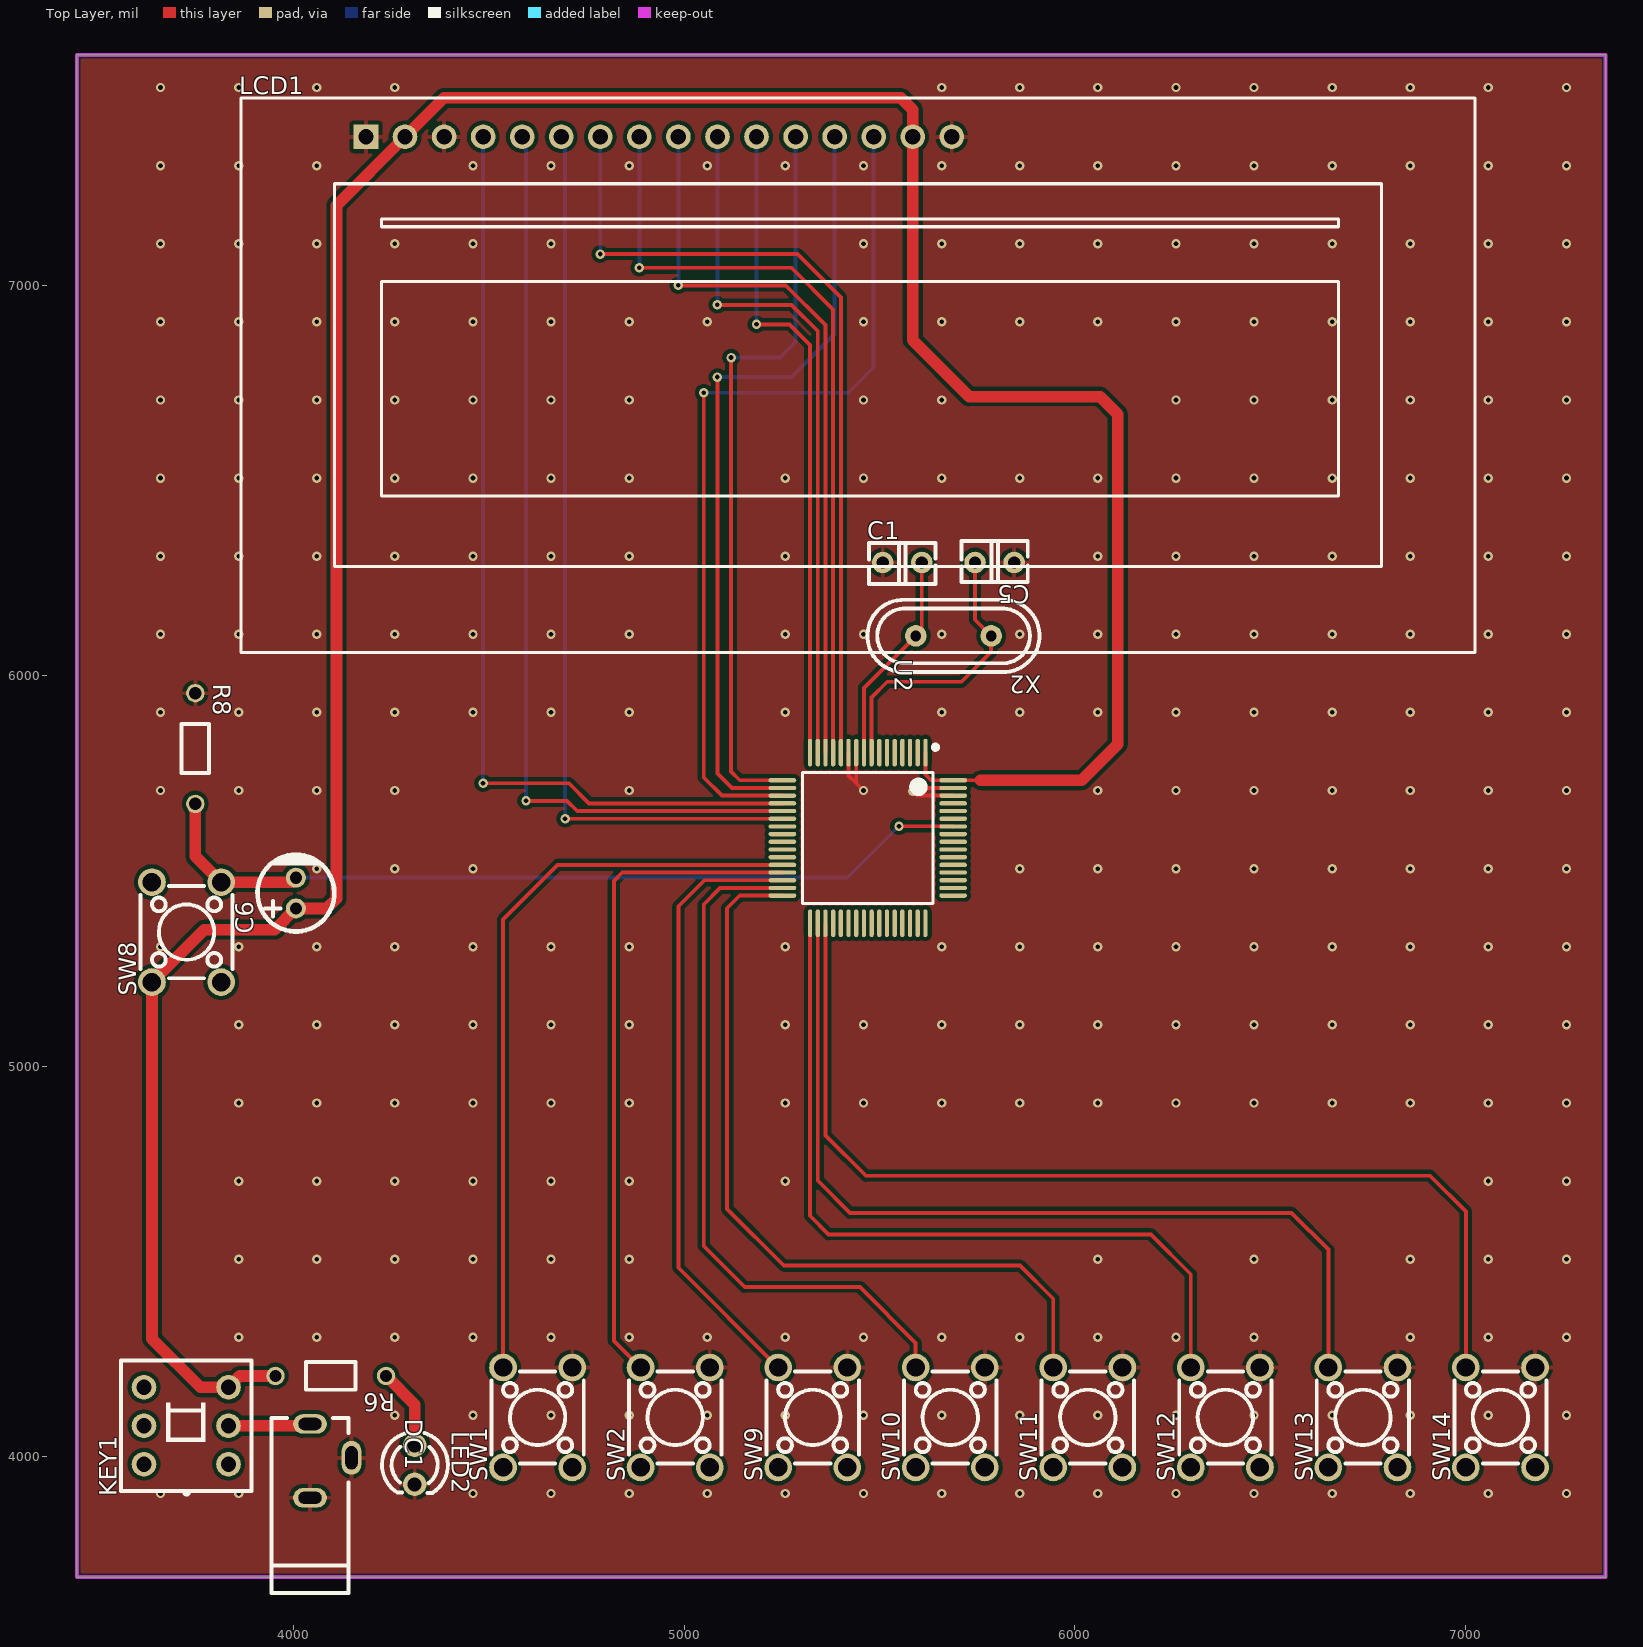
[diagram p0: Top Layer view]
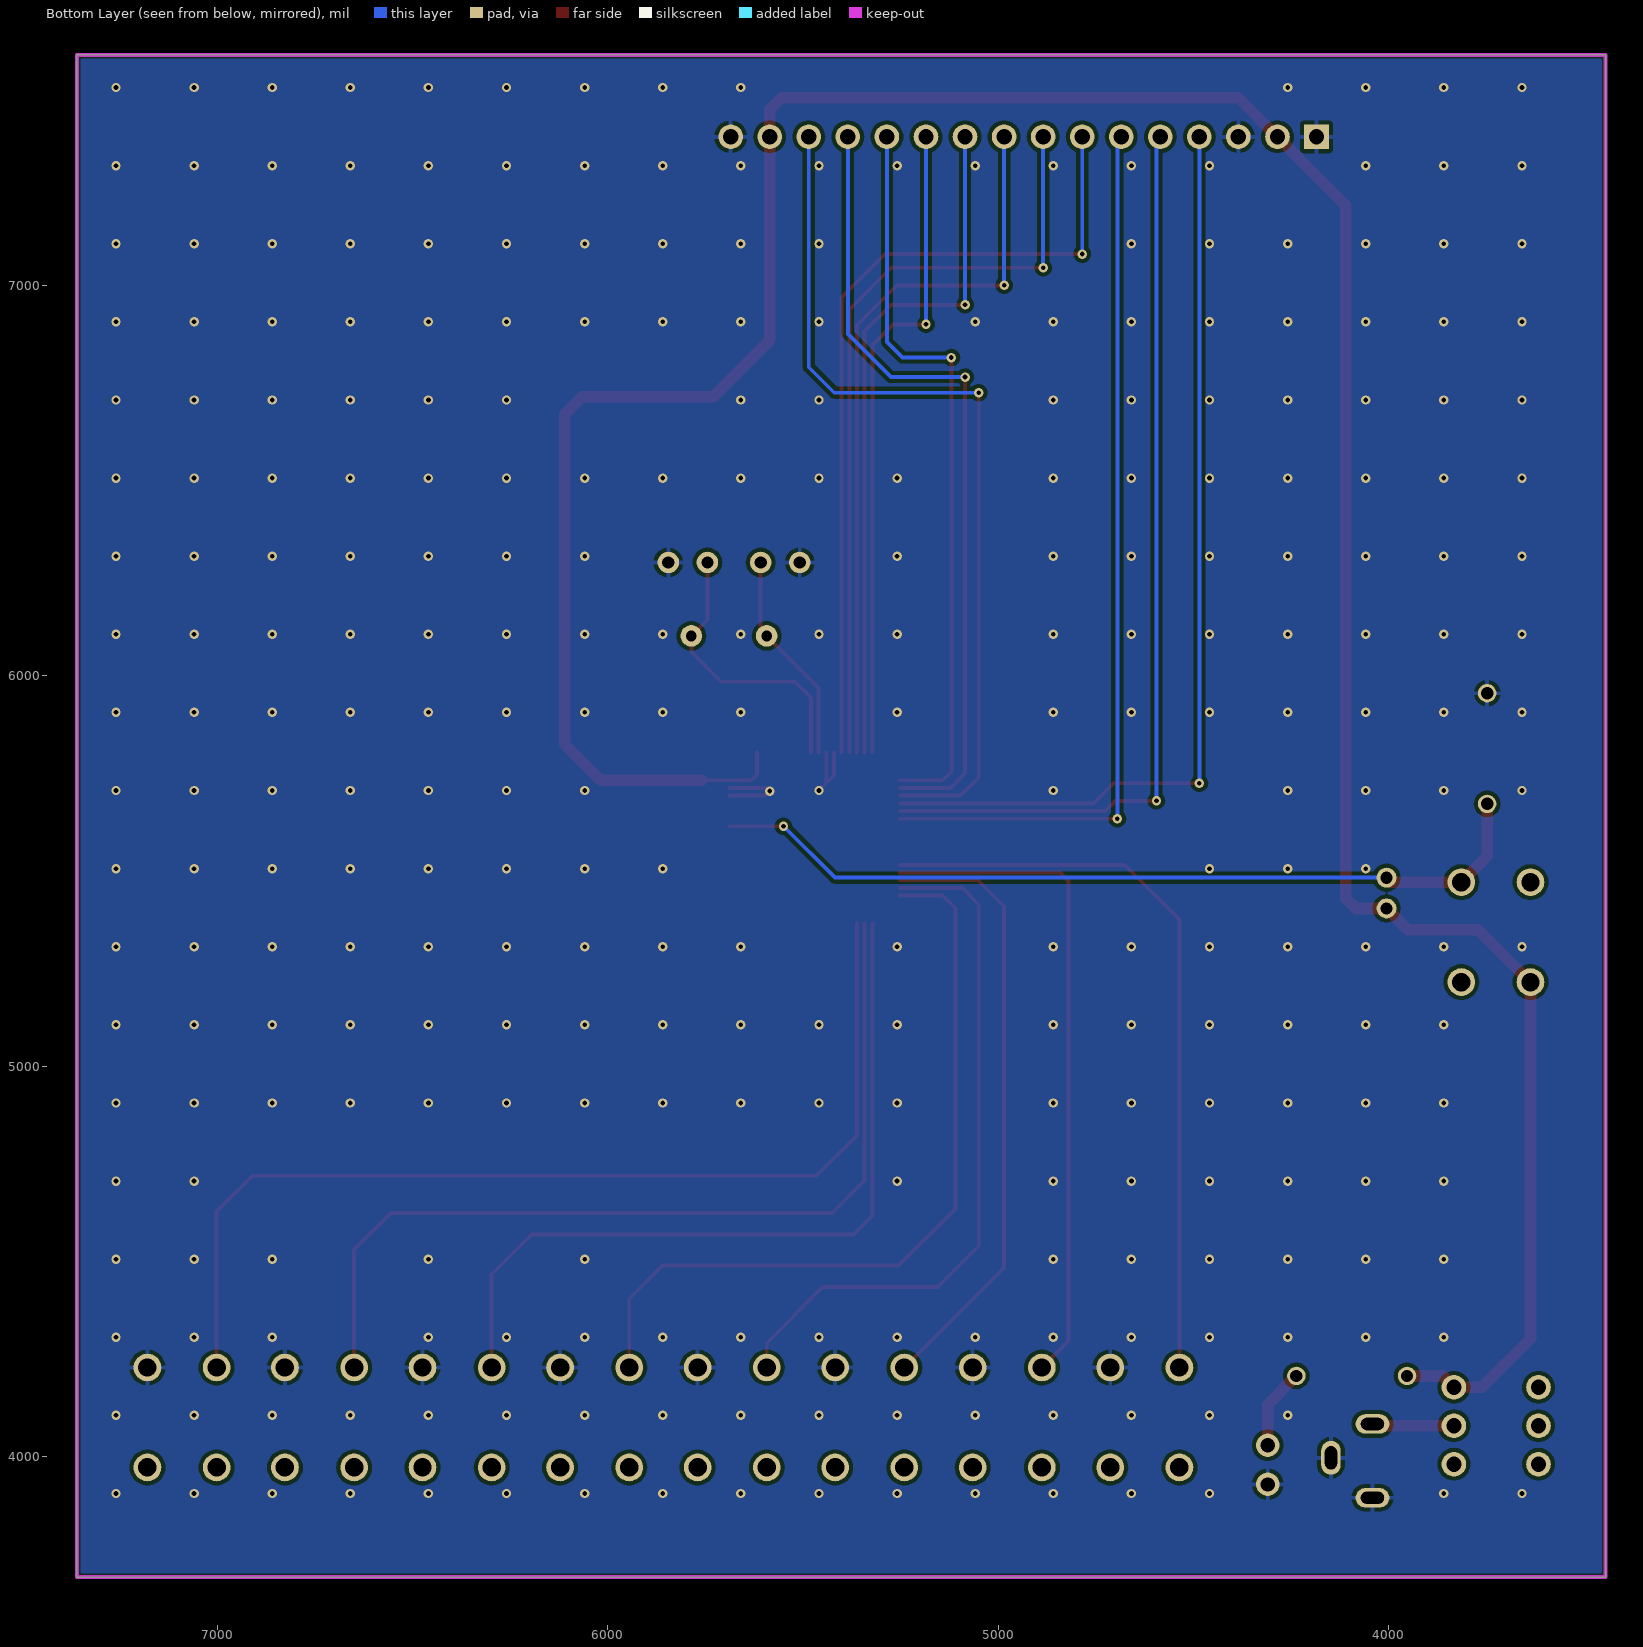
[diagram p1: Bottom Layer view, seen from below]
# Altium PCB MISC51174.pcbdoc
Units mil, origin at the board's own origin, x right, y up, seen from the top; angles counter-clockwise.
Board outline 3914.17 x 3897.64 mil, 2 copper layers (Top Layer, Bottom Layer), stack 62.206 mil thick; 20 components, 26 nets, 139 pads, 306 vias.

## Layer stack, top to bottom
Top Solder Mask Layer: solder mask 0.394, Dk 3.3
Top Layer: signal copper 1.379
Dielectric1: surface 59.449, FR4, Dk 4.5
Bottom Layer: signal copper 1.378
Bottom Solder Mask Layer: solder mask 0.394, Dk 3.3

## Board outline
3445,7590 3445,3692.36 7359.17,3692.36 7359.17,7590

## Design rules (kind name [scope] priority, off if disabled: settings)
BoardOutlineClearance copperThickness2oz_1 [All] p2 off: genericclearance=7.99 ignorepadtopadclearanceinfootprint=FALSE except(0: Arc-SplitContinuation Track-SplitContinuation SMDPad-SplitContinuation THPad-SplitContinuation Via-SplitContinuation Fill-SplitContinuation Region-SplitContinuation Poly-SplitContinuation Text-SplitContinuation Hole-SplitContinuation; 5.98: Arc-CutoutEdge SMDPad-CutoutEdge THPad-CutoutEdge Via-CutoutEdge Fill-CutoutEdge Region-CutoutEdge Text-CutoutEdge; 6.93: Hole-OutlineEdge Hole-CutoutEdge; 10: Poly-OutlineEdge Poly-CutoutEdge; 11.81: Arc-OutlineEdge Track-OutlineEdge SMDPad-OutlineEdge THPad-OutlineEdge Via-OutlineEdge Fill-OutlineEdge Region-OutlineEdge Text-OutlineEdge Track-CutoutEdge)
BoardOutlineClearance copperThickness1oz_1 [All] p4: genericclearance=4.02 ignorepadtopadclearanceinfootprint=FALSE except(0: Arc-SplitContinuation Track-SplitContinuation SMDPad-SplitContinuation THPad-SplitContinuation Via-SplitContinuation Fill-SplitContinuation Region-SplitContinuation Poly-SplitContinuation Text-SplitContinuation Hole-SplitContinuation; 6: SMDPad-CutoutEdge THPad-CutoutEdge Via-CutoutEdge Fill-CutoutEdge Region-CutoutEdge Text-CutoutEdge; 6.93: Hole-OutlineEdge Hole-CutoutEdge; 10: Poly-OutlineEdge Poly-CutoutEdge; 11.8: Arc-OutlineEdge Track-OutlineEdge SMDPad-OutlineEdge THPad-OutlineEdge Via-OutlineEdge Fill-OutlineEdge Region-OutlineEdge Text-OutlineEdge; 11.81: Arc-CutoutEdge Track-CutoutEdge)
Clearance copperThickness2oz [All] p1 off: gap=7.99 ignorepadtopadclearanceinfootprint=FALSE except(5.98: SMDPad-Track SMDPad-SMDPad THPad-Track SMDPad-THPad THPad-THPad Track-Via SMDPad-Via THPad-Via Via-Via Fill-Track Region-Track Fill-SMDPad Region-SMDPad Fill-THPad Region-THPad Fill-Via Region-Via Fill-Fill Fill-Region Region-Region Arc-Track Arc-SMDPad Arc-THPad Arc-Via Fill-Arc Region-Arc Arc-Arc Text-Track SMDPad-Text Text-THPad Text-Via Fill-Text Region-Text Arc-Text Text-Text; 6.93: Hole-Track Hole-SMDPad Hole-THPad Hole-Via Fill-Hole Region-Hole Hole-Arc Hole-Text; 10: Poly-Track Poly-SMDPad Poly-THPad Poly-Via Poly-Fill Poly-Region Poly-Poly Poly-Arc Poly-Text Poly-Hole)
Clearance copperThickness1oz [All] p3: gap=4.02 ignorepadtopadclearanceinfootprint=FALSE except(5.98: SMDPad-Track SMDPad-SMDPad THPad-Track SMDPad-THPad THPad-THPad Track-Via SMDPad-Via THPad-Via Via-Via Fill-Track Region-Track Fill-SMDPad Region-SMDPad Fill-THPad Region-THPad Fill-Via Region-Via Fill-Fill Fill-Region Region-Region; 6: Arc-Track Arc-SMDPad Arc-THPad Arc-Via Fill-Arc Region-Arc Arc-Arc Text-Track SMDPad-Text Text-THPad Text-Via Fill-Text Region-Text Arc-Text Text-Text; 6.93: Hole-Track Hole-SMDPad Hole-THPad Hole-Via Fill-Hole Region-Hole Hole-Arc Hole-Text; 10: Poly-Track Poly-SMDPad Poly-THPad Poly-Via Poly-Fill Poly-Region Poly-Poly Poly-Arc Poly-Text Poly-Hole)
Creepage creepage [All] p1: checkdistance=0 ignoreinternallayers=TRUE applytopolygonpour=TRUE
DiffPairsRouting differentialPair [All] p1: maxlimit=6 minlimit=6 mostfreqgap=6 toplayer_minwidth=5 toplayer_prefwidth=10 toplayer_maxwidth=100 toplayer_mingap=6 toplayer_prefgap=6 toplayer_maxgap=6 bottomlayer_minwidth=5 bottomlayer_prefwidth=10 bottomlayer_maxwidth=100 bottomlayer_mingap=6 bottomlayer_prefgap=6 bottomlayer_maxgap=6 maxuncoupledlength=10
HoleToHoleClearance otherClearance [All] p1: gap=11.81 allowstackedmicrovias=TRUE
Length netLength [All] p1: minlimit=0 maxlimit=0
MatchedLengths netLengthTolerance [All] p1: tolerance=1000
PasteMaskExpansion pasteMaskExpansion [All] p1: expansion=0
PlaneConnect innerPlane [All] p1: planeconnectstyle=Relief reliefexpansion=20 reliefentries=4 reliefconductorwidth=10 reliefairgap=10
PolygonConnect copperRegion [(InNet('GND'))] p1: connectstyle=Relief reliefconductorwidth=10 reliefentries=4 polygonreliefangle="90 Angle" airgapwidth=10 via.connectstyle=Relief via.reliefconductorwidth=10 via.reliefentries=4 via.polygonreliefangle="90 Angle" via.airgapwidth=10
RoutingVias viaSize [All] p1: holewidth=12.01 width=24.02 viastyle="Through Hole" minholewidth=11.81 minwidth=19.68 maxholewidth=248.03 maxwidth=393.7
SolderMaskExpansion solderMaskExpansion [IsVia] p1: expansion=-1000 istentingtop=TRUE
SolderMaskExpansion solderMaskExpansion [All] p2: expansion=2 istentingtop=FALSE
Width copperThickness2oz_2 [All] p1 off: maxlimit=100 minlimit=8 preferedwidth=10
Width copperThickness1oz_2 [All] p2: maxlimit=100 minlimit=5 preferedwidth=10

## Components (designator, comment, footprint, x,y, rotation, side; value= is the part's Value field where it differs from the comment)
C1 "30pF" CAP-TH_L3.8-W2.5-P2.54-D0.50 5558.34,6290.38 r0 top
C5 "30pF" CAP-TH_L3.8-W2.5-P2.54-D0.50 5794.74,6290.39 r180 top
C6 "10uF" CAP-TH_BD5.0-P2.00-D0.8-FD-10UF50VC110GL 4005.8,5443.88 r90 top
DC1 "DC-002" DC-IN-TH_DC-3510 4095,3990 r270 top
KEY1 "Non-latching switch 8.5×8.5 silent" SW-TH_6P-L8.5-W8.5-P2.54 3725,4080 r90 top
LCD1 "LCD1602" LCD1602 5445,6770 r0 top
LED2 "" LED_TH-3mm 4310,3980 r270 top
R6 "1kΩ" Res_1/8W 4095,4210 r180 top
R8 "10kΩ" Res_1/8W 3745.8,5813.88 r270 top
SW1 "" SW-TH_4P-L6.0-W6.0-P4.50-LS6.5 4624.72,4101.14 r90 top
SW2 "" SW-TH_4P-L6.0-W6.0-P4.50-LS6.5 4976.91,4101.14 r90 top
SW8 "" SW-TH_4P-L6.0-W6.0-P4.50-LS6.5 3725.8,5343.88 r90 top
SW9 "" SW-TH_4P-L6.0-W6.0-P4.50-LS6.5 5329.09,4101.14 r90 top
SW10 "" SW-TH_4P-L6.0-W6.0-P4.50-LS6.5 5681.27,4101.14 r90 top
SW11 "" SW-TH_4P-L6.0-W6.0-P4.50-LS6.5 6033.45,4101.14 r90 top
SW12 "" SW-TH_4P-L6.0-W6.0-P4.50-LS6.5 6385.64,4101.14 r90 top
SW13 "" SW-TH_4P-L6.0-W6.0-P4.50-LS6.5 6737.82,4101.14 r90 top
SW14 "" SW-TH_4P-L6.0-W6.0-P4.50-LS6.5 7090,4101.14 r90 top
U2 "MSP430F2491TPM" LQFP-64_L10.0-W10.0-P0.50-LS12.0-TL 5470,5585 r270 top
X2 "11.0592MHz" OSC-TH_L11.1-W4.7-P4.88 5689.54,6102.36 r180 top

## Footprints (in the part's own frame and the unit in brackets; to place one, negate y for a bottom-side part, rotate by r counter-clockwise, add the part's x,y. Pads: shape width x height; smd on the part's side, far side on the other; paste and mask are expansions set on the pad)
CAP-TH_BD5.0-P2.00-D0.8-FD-10UF50VC110GL [mm]
  round 1.3 hole 0.8: 1(-1,0) 2(1,0)
  silkscreen extent -2.5,-2.5 2.5,2.5
CAP-TH_L3.8-W2.5-P2.54-D0.50 [mm]
  round 1.4 hole 0.8 paste+0 mask+0.05: 1(-1.27,0) 2(1.27,0)
  silkscreen extent -2.16,-1.4 2.16,1.27
DC-IN-TH_DC-3510 [mm]
  oval 1.27x2.2 hole 0.8 slot 1.5 at 90 deg: 1(-2.4,-1.35) 2(2.4,-1.35)
  oval 2.2x1.27 hole 0.8 slot 1.5 at 0 deg: 3(-0.2,1.35)
  silkscreen extent -2.8,-3.85 8.6,1.15
LCD1602 [mm]
  rect 1.6x1.6 hole 1: 1(-32,15.5)
  round 1.6 hole 1: 2(-29.46,15.5) 3(-26.92,15.5) 4(-24.38,15.5) 5(-21.84,15.5) 6(-19.3,15.5) 7(-16.76,15.5) 8(-14.22,15.5) 9(-11.68,15.5) 10(-9.14,15.5) 11(-6.6,15.5) 12(-4.06,15.5) 13(-1.52,15.5) 14(1.02,15.5) 15(3.56,15.5) 16(6.1,15.5)
  silkscreen extent -40.13,-18.03 40.13,18.03
LED_TH-3mm [mil]
  round 60 hole 36 paste+0 mask+2: 1(-50,0) 2(50,0)
  silkscreen extent -81,-84 72,85
LQFP-64_L10.0-W10.0-P0.50-LS12.0-TL [mm]
  oval 1.8x0.28 smd paste+0 mask+0.05: 1(-5.55,3.75) 2(-5.55,3.25) 3(-5.55,2.75) 4(-5.55,2.25) 5(-5.55,1.75) 6(-5.55,1.25) 7(-5.55,0.75) 8(-5.55,0.25) 9(-5.55,-0.25) 10(-5.55,-0.75) 11(-5.55,-1.25) 12(-5.55,-1.75) 13(-5.55,-2.25) 14(-5.55,-2.75) 15(-5.55,-3.25) 16(-5.55,-3.75) 33(5.55,-3.75) 34(5.55,-3.25) 35(5.55,-2.75) 36(5.55,-2.25) 37(5.55,-1.75) 38(5.55,-1.25) 39(5.55,-0.75) 40(5.55,-0.25) 41(5.55,0.25) 42(5.55,0.75) 43(5.55,1.25) 44(5.55,1.75) 45(5.55,2.25) 46(5.55,2.75) 47(5.55,3.25) 48(5.55,3.75)
  oval 0.28x1.8 smd paste+0 mask+0.05: 17(-3.75,-5.55) 18(-3.25,-5.55) 19(-2.75,-5.55) 20(-2.25,-5.55) 21(-1.75,-5.55) 22(-1.25,-5.55) 23(-0.75,-5.55) 24(-0.25,-5.55) 25(0.25,-5.55) 26(0.75,-5.55) 27(1.25,-5.55) 28(1.75,-5.55) 29(2.25,-5.55) 30(2.75,-5.55) 31(3.25,-5.55) 32(3.75,-5.55) 49(3.75,5.55) 50(3.25,5.55) 51(2.75,5.55) 52(2.25,5.55) 53(1.75,5.55) 54(1.25,5.55) 55(0.75,5.55) 56(0.25,5.55) 57(-0.25,5.55) 58(-0.75,5.55) 59(-1.25,5.55) 60(-1.75,5.55) 61(-2.25,5.55) 62(-2.75,5.55) 63(-3.25,5.55) 64(-3.75,5.55)
  silkscreen extent -6.05,-4.25 4.25,4.55
OSC-TH_L11.1-W4.7-P4.88 [mm]
  round 1.4 hole 0.7: 1(-2.45,0) 2(2.45,0)
  silkscreen extent -5.59,-2.35 5.6,2.35
Res_1/8W [mil]
  round 47.2 hole 31.5 paste+0 mask+2: 1(-141.7,2.48) 2(141.7,2.48)
  silkscreen extent -63,-33 63,38
SW-TH_4P-L6.0-W6.0-P4.50-LS6.5 [mm]
  round 1.8 hole 1.2: 1(-3.25,2.25) 2(3.25,2.25) 3(-3.25,-2.25) 4(3.25,-2.25)
  silkscreen extent -3,-3 3,3
SW-TH_6P-L8.5-W8.5-P2.54 [mm]
  round 1.6 hole 1: 1(-2.5,-2.75) 2(0,-2.75) 3(2.5,-2.75) 4(-2.5,2.75) 5(0,2.75) 6(2.5,2.75)
  silkscreen extent -4.47,-4.25 4.25,4.25

## Via types
v1: diameter 24.02, hole 12, Top Layer to Bottom Layer, 306 vias

## Nets (pads, with @x,y where several pads share a name; then routed paths per layer and width w, separated by ;. In a path a pad name is that pad's centre, name@x,y a point inside that pad or via, vN(x,y) a via of type N, cw(c..) or ccw(c..) an arc to the next point about the centre after c; other vN are vias at no path point)
$1N111: LED2.1 R6.1 | length 207.9
  Top Layer w30: R6.1 4310,4134.22 LED2.1
$1N113: DC1.1 KEY1.2 | length 210.4
  Top Layer w30: KEY1.2 4037.36,4079.99 DC1.1
GND: C1.1 C5.1 DC1.2 DC1.3 LCD1.1 LCD1.3 LCD1.16 LED2.2 R8.1 SW1.4 SW2.4 SW9.4 SW10.4 SW11.4 SW12.4 SW13.4 SW14.4 U2.10 U2.11 U2.62 U2.63 | length 406.5
  Top Layer w10: U2.11 5420.79,5744.77 5440.47,5725.09 ; U2.10 5440.47,5725.09 ; v1(5459.1,5706.46) 5440.47,5725.09 ; U2.62 5596.73,5693.27 v1(5585,5705) 5592.95,5712.95 U2.63
  other v1: 3659.1,3906.46 3859.1,3906.46 4459.1,3906.46 4659.1,3906.46 4859.1,3906.46 5059.1,3906.46 5259.1,3906.46 5459.1,3906.46 5659.1,3906.46 5859.1,3906.46 6059.1,3906.46 6259.1,3906.46 6459.1,3906.46 6659.1,3906.46 6859.1,3906.46 7059.1,3906.46 7259.1,3906.46 4259.1,4106.46 4459.1,4106.46 4659.1,4106.46 4859.1,4106.46 5059.1,4106.46 5259.1,4106.46 5459.1,4106.46 5659.1,4106.46 5859.1,4106.46 6059.1,4106.46 6259.1,4106.46 6459.1,4106.46 6659.1,4106.46 6859.1,4106.46 7059.1,4106.46 7259.1,4106.46 3859.1,4306.46 4059.1,4306.46 4259.1,4306.46 4459.1,4306.46 4659.1,4306.46 4859.1,4306.46 5059.1,4306.46 5259.1,4306.46 5459.1,4306.46 5659.1,4306.46 5859.1,4306.46 6059.1,4306.46 6259.1,4306.46 6459.1,4306.46 6859.1,4306.46 7059.1,4306.46 7259.1,4306.46 3859.1,4506.46 4059.1,4506.46 4259.1,4506.46 4459.1,4506.46 4659.1,4506.46 4859.1,4506.46 6059.1,4506.46 6459.1,4506.46 6859.1,4506.46 7059.1,4506.46 7259.1,4506.46 3859.1,4706.46 4059.1,4706.46 4259.1,4706.46 4459.1,4706.46 4659.1,4706.46 4859.1,4706.46 5259.1,4706.46 7059.1,4706.46 7259.1,4706.46 3859.1,4906.46 4059.1,4906.46 4259.1,4906.46 4459.1,4906.46 4659.1,4906.46 4859.1,4906.46 5259.1,4906.46 5459.1,4906.46 5659.1,4906.46 5859.1,4906.46 6059.1,4906.46 6259.1,4906.46 6459.1,4906.46 6659.1,4906.46 6859.1,4906.46 7059.1,4906.46 7259.1,4906.46 3859.1,5106.46 4059.1,5106.46 4259.1,5106.46 4459.1,5106.46 4659.1,5106.46 4859.1,5106.46 5259.1,5106.46 5459.1,5106.46 5659.1,5106.46 5859.1,5106.46 6059.1,5106.46 6259.1,5106.46 6459.1,5106.46 6659.1,5106.46 6859.1,5106.46 7059.1,5106.46 7259.1,5106.46 3659.1,5306.46 3859.1,5306.46 4059.1,5306.46 4259.1,5306.46 4459.1,5306.46 4659.1,5306.46 4859.1,5306.46 5259.1,5306.46 5659.1,5306.46 5859.1,5306.46 6059.1,5306.46 6259.1,5306.46 6459.1,5306.46 6659.1,5306.46 6859.1,5306.46 7059.1,5306.46 7259.1,5306.46 4059.1,5506.46 4259.1,5506.46 4459.1,5506.46 5859.1,5506.46 6059.1,5506.46 6259.1,5506.46 6459.1,5506.46 6659.1,5506.46 6859.1,5506.46 7059.1,5506.46 7259.1,5506.46 3659.1,5706.46 3859.1,5706.46 4059.1,5706.46 4259.1,5706.46 4859.1,5706.46 6059.1,5706.46 6259.1,5706.46 6459.1,5706.46 6659.1,5706.46 6859.1,5706.46 7059.1,5706.46 7259.1,5706.46 3659.1,5906.46 3859.1,5906.46 4059.1,5906.46 4259.1,5906.46 4459.1,5906.46 4659.1,5906.46 4859.1,5906.46 5259.1,5906.46 5659.1,5906.46 5859.1,5906.46 6059.1,5906.46 6259.1,5906.46 6459.1,5906.46 6659.1,5906.46 6859.1,5906.46 7059.1,5906.46 7259.1,5906.46 3659.1,6106.46 3859.1,6106.46 4059.1,6106.46 4259.1,6106.46 4459.1,6106.46 4659.1,6106.46 4859.1,6106.46 5259.1,6106.46 5459.1,6106.46 5659.1,6106.46 5859.1,6106.46 6059.1,6106.46 6259.1,6106.46 6459.1,6106.46 6659.1,6106.46 6859.1,6106.46 7059.1,6106.46 7259.1,6106.46 3659.1,6306.46 3859.1,6306.46 4059.1,6306.46 4259.1,6306.46 4459.1,6306.46 4659.1,6306.46 4859.1,6306.46 5259.1,6306.46 6059.1,6306.46 6259.1,6306.46 6459.1,6306.46 6659.1,6306.46 6859.1,6306.46 7059.1,6306.46 7259.1,6306.46 3659.1,6506.46 3859.1,6506.46 4059.1,6506.46 4259.1,6506.46 4459.1,6506.46 4659.1,6506.46 4859.1,6506.46 5259.1,6506.46 5459.1,6506.46 5659.1,6506.46 5859.1,6506.46 6059.1,6506.46 6259.1,6506.46 6459.1,6506.46 6659.1,6506.46 6859.1,6506.46 7059.1,6506.46 7259.1,6506.46 3659.1,6706.46 3859.1,6706.46 4059.1,6706.46 4259.1,6706.46 4459.1,6706.46 4659.1,6706.46 4859.1,6706.46 5459.1,6706.46 5659.1,6706.46 6259.1,6706.46 6459.1,6706.46 6659.1,6706.46 6859.1,6706.46 7059.1,6706.46 7259.1,6706.46 3659.1,6906.46 3859.1,6906.46 4059.1,6906.46 4259.1,6906.46 4459.1,6906.46 4659.1,6906.46 4859.1,6906.46 5059.1,6906.46 5459.1,6906.46 5659.1,6906.46 5859.1,6906.46 6059.1,6906.46 6259.1,6906.46 6459.1,6906.46 6659.1,6906.46 6859.1,6906.46 7059.1,6906.46 7259.1,6906.46 3659.1,7106.46 3859.1,7106.46 4059.1,7106.46 4259.1,7106.46 4459.1,7106.46 4659.1,7106.46 5459.1,7106.46 5659.1,7106.46 5859.1,7106.46 6059.1,7106.46 6259.1,7106.46 6459.1,7106.46 6659.1,7106.46 6859.1,7106.46 7059.1,7106.46 7259.1,7106.46 3659.1,7306.46 3859.1,7306.46 4059.1,7306.46 4459.1,7306.46 4659.1,7306.46 4859.1,7306.46 5059.1,7306.46 5259.1,7306.46 5459.1,7306.46 5659.1,7306.46 5859.1,7306.46 6059.1,7306.46 6259.1,7306.46 6459.1,7306.46 6659.1,7306.46 6859.1,7306.46 7059.1,7306.46 7259.1,7306.46 3659.1,7506.46 3859.1,7506.46 4059.1,7506.46 4259.1,7506.46 5659.1,7506.46 5859.1,7506.46 6059.1,7506.46 6259.1,7506.46 6459.1,7506.46 6659.1,7506.46 6859.1,7506.46 7059.1,7506.46 7259.1,7506.46
P10: LCD1.7 U2.12 | length 2127.8
  Top Layer w10: v1(4785,7080) 5290,7080 5401.1,6968.9 U2.12
  Bottom Layer w10: v1(4785,7080) 4785,7380.08 LCD1.7
P11: LCD1.8 U2.13 | length 2010.7
  Top Layer w10: v1(4885.16,7045) 5275,7045 5381.42,6938.58 U2.13
  Bottom Layer w10: v1(4885.16,7045) LCD1.8
P12: LCD1.9 U2.14 | length 1893.9
  Top Layer w10: v1(4985,7000) 5260,7000 5361.73,6898.27 U2.14
  Bottom Layer w10: v1(4985,7000) 4985,7380.08 LCD1.9
P13: LCD1.10 U2.15 | length 1794.6
  Top Layer w10: v1(5085,6950) 5275,6950 5342.05,6882.95 U2.15
  Bottom Layer w10: v1(5085,6950) 5085,7380.08 LCD1.10
P14: LCD1.11 U2.16 | length 1683.5
  Top Layer w10: v1(5185,6900) 5270,6900 5322.36,6847.64 U2.16
  Bottom Layer w10: v1(5185,6900) 5185,7380.08 LCD1.11
P15: LCD1.12 U2.17 | length 1907.6
  Top Layer w10: v1(5120,6815) 5120,5755 5142.36,5732.64 U2.17
  Bottom Layer w10: v1(5120,6815) 5245,6815 5285,6855 5285,7380.08 LCD1.12
P16: LCD1.13 U2.18 | length 2047.7
  Top Layer w10: v1(5085,6765) 5085,5750 5122.05,5712.95 U2.18
  Bottom Layer w10: v1(5085,6765) 5275,6765 5385.16,6875.16 LCD1.13
P17: LCD1.14 U2.19 | length 2258.1
  Top Layer w10: v1(5050,6725) 5050,5740 5096.73,5693.27 U2.19
  Bottom Layer w10: v1(5050,6725) 5420,6725 5485.16,6790.16 LCD1.14
P20: LCD1.4 U2.20 | length 2443.1
  Top Layer w10: v1(4485,5725) 4705,5725 4756.42,5673.58 U2.20
  Bottom Layer w10: v1(4485,5725) 4485,7380.08 LCD1.4
P21: LCD1.5 U2.21 | length 2371.6
  Top Layer w10: v1(4595,5680) 4700,5680 4726.1,5653.9 U2.21
  Bottom Layer w10: LCD1.5 4595,7370.4 v1(4595,5680)
P22: LCD1.6 U2.22 | length 2306.6
  Top Layer w10: v1(4695,5634.21) U2.22
  Bottom Layer w10: LCD1.6 4695,7370.4 v1(4695,5634.21)
P30: SW1.2 U2.28 | length 1920.4
  Top Layer w10: SW1.2 4536.14,5376.14 4676.1,5516.1 U2.28
P31: SW2.2 U2.29 | length 1714.6
  Top Layer w10: SW2.2 4820,4297.42 4820,5475 4841.42,5496.42 U2.29
P32: SW9.2 U2.30 | length 1580.9
  Top Layer w10: SW9.2 4985,4484.6 4985,5410 5051.73,5476.73 U2.30
P33: SW10.2 U2.31 | length 1802.4
  Top Layer w10: U2.31 5092.05,5457.05 5050,5415 5050,4540 5155,4435 5450,4435 5592.69,4292.31 SW10.2
P34: SW11.2 U2.32 | length 2031
  Top Layer w10: U2.32 5142.36,5437.36 5110,5405 5110,4635 5255,4490 5860,4490 5944.87,4405.13 SW11.2
P35: SW12.2 U2.33 | length 2024.4
  Top Layer w10: U2.33 5322.36,4617.64 5370,4570 6195,4570 6297.06,4467.94 SW12.2
P36: SW13.2 U2.34 | length 2340.8
  Top Layer w10: U2.34 5342.05,4707.95 5425,4625 6555,4625 6649.24,4530.76 SW13.2
P37: SW14.2 U2.35 | length 2663.1
  Top Layer w10: U2.35 5361.73,4823.27 5465,4720 6910,4720 7001.42,4628.58 SW14.2
RST: C6.2 R8.2 SW8.4 U2.58 | length 2161.4
  Top Layer w10: v1(5550,5615) 5688.03,5615 U2.58
  Top Layer w30: R8.2 3748.27,5537.93 SW8.4 3994.38,5471.83 C6.2
  Bottom Layer w10: C6.2 5418.25,5483.25 v1(5550,5615)
VCC: C6.1 KEY1.3 LCD1.2 LCD1.15 R6.2 SW8.1 U2.1 U2.64 | length 7862.2
  Top Layer w10: U2.1 5617.64,5747.36 5632.36,5732.64 U2.64 5758.93,5732.64
  Top Layer w30: R6.2 3862.37,4207.52 KEY1.3 3761.57,4178.43 3637.22,4302.78 SW8.1 3771.29,5350 3951.29,5350 C6.1 4084.51,5404.51 4110,5430 4110,7205.08 LCD1.2 4384.92,7480 5555,7480 5585.16,7449.84 LCD1.15 5585.16,6859.84 5730,6715 6065,6715 6110,6670 6110,5825 6017.64,5732.64 5758.93,5732.64
X1: C5.2 U2.8 X2.1 | length 742.1
  Top Layer w10: U2.8 5479.84,5944.84 5520,5985 5710,5985 5785.99,6060.99 X2.1 5744.74,6143.6 C5.2
X2: C1.2 U2.9 X2.2 | length 548.3
  Top Layer w10: U2.9 5460.16,5969.43 X2.2 5608.34,6117.61 C1.2
pads on no net: KEY1.1 KEY1.4 KEY1.5 KEY1.6 SW1.1 SW1.3 SW2.1 SW2.3 SW8.2 SW8.3 SW9.1 SW9.3 SW10.1 SW10.3 SW11.1 SW11.3 SW12.1 SW12.3 SW13.1 SW13.3 SW14.1 SW14.3 U2.2 U2.3 U2.4 U2.5 U2.6 U2.7 U2.23 U2.24 U2.25 U2.26 U2.27 U2.36 U2.37 U2.38 U2.39 U2.40 U2.41 U2.42 U2.43 U2.44 U2.45 U2.46 U2.47 U2.48 U2.49 U2.50 U2.51 U2.52 U2.53 U2.54 U2.55 U2.56 U2.57 U2.59 U2.60 U2.61

## Polygon pours and split planes (outlines as drawn)
GND on Top Layer (solid, remove dead copper, pour order 0): 3020,7875 3020,3000 7830,3000 7830,7875
GND on Bottom Layer (solid, remove dead copper, pour order 2): 3000,7800 3000,3185 7995,3185 7995,7800

## Keep-outs
Board Outline Layer:
  the board outline again, w10